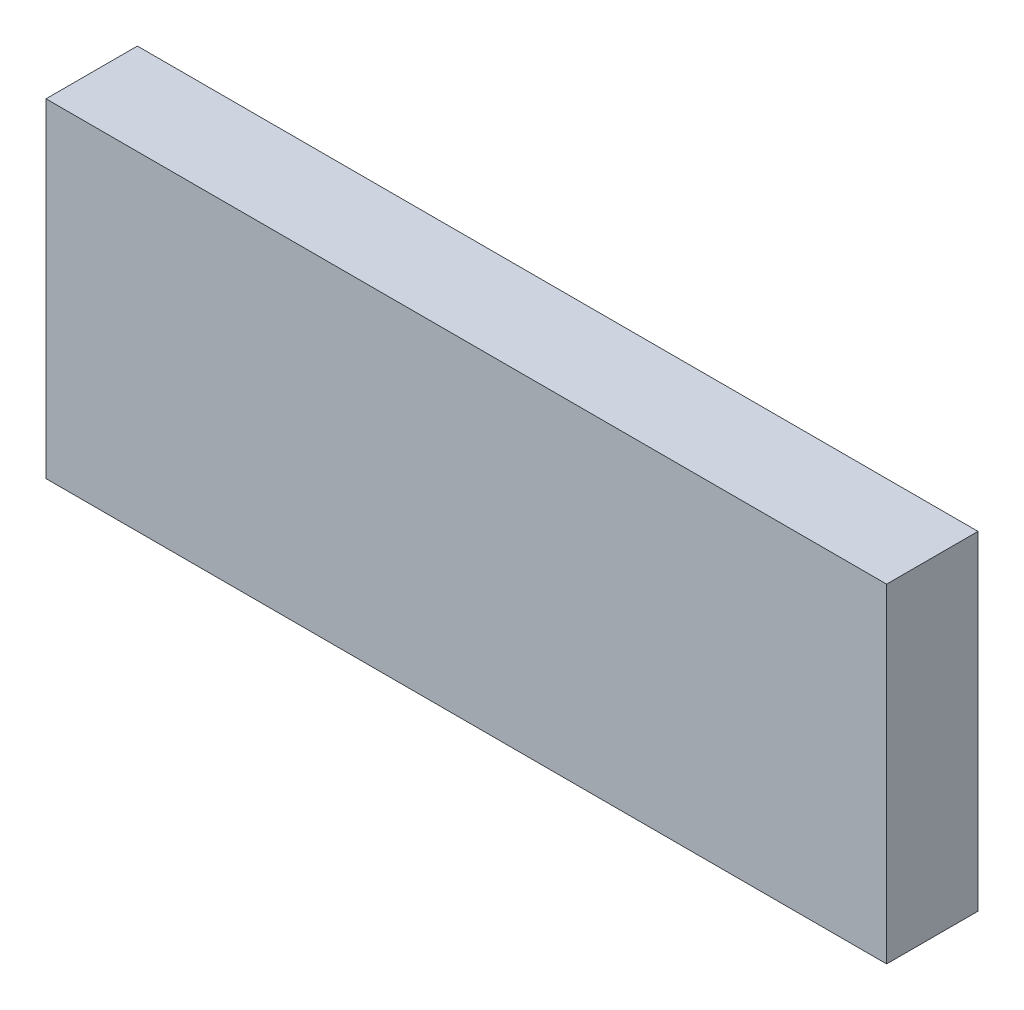
SolidWorks part; units mm, degrees
ref_plane "Front Plane" through (0, 0, 0) normal (0, 0, 1) x (1, 0, 0)
ref_plane "Top Plane" through (0, 0, 0) normal (0, 1, 0) x (1, 0, 0)
ref_plane "Right Plane" through (0, 0, 0) normal (1, 0, 0) x (0, 0, -1)
sketch "Sketch1" plane through (0, 0, 0) normal (0, 0, 1) x (1, 0, 0)
  line L1 (0, 0) -> (-230, 0)
  line L2 (0, 0) -> (0, 90)
  line L3 (0, 90) -> (-230, 90)
  line L4 (-230, 0) -> (-230, 90)
  dimension "D1" = 230
  dimension "D2" = 90
extrude "Boss-Extrude1" add sketch "Sketch1" along normal blind 25
